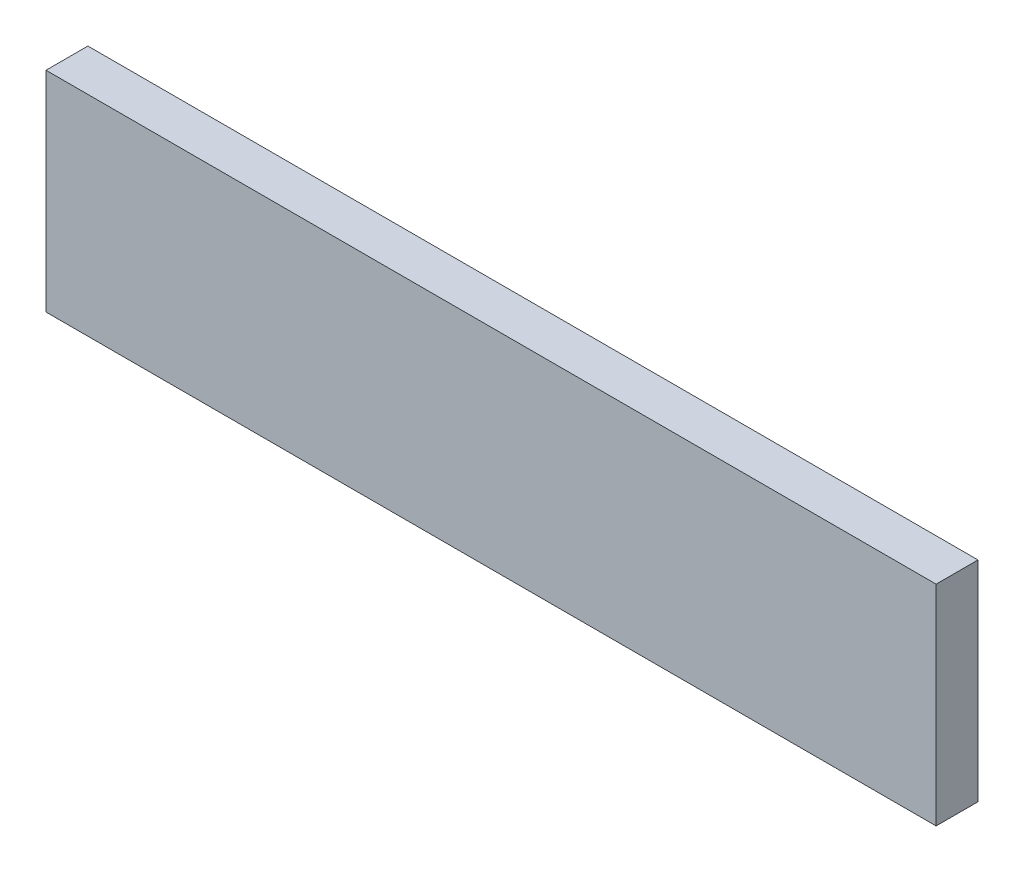
from build123d import *

# Parameters (mm, degrees)
SKETCH1_W           = 425
SKETCH1_H           = 100
BOSS_EXTRUDE1_DEPTH = 20


with BuildPart() as part:
    # Sketch1 → Boss-Extrude1 (new body)
    with BuildSketch(Plane.XY):
        with Locations((212.5, 50)):
            Rectangle(SKETCH1_W, SKETCH1_H)
    extrude(amount=BOSS_EXTRUDE1_DEPTH)


solid = part.part
